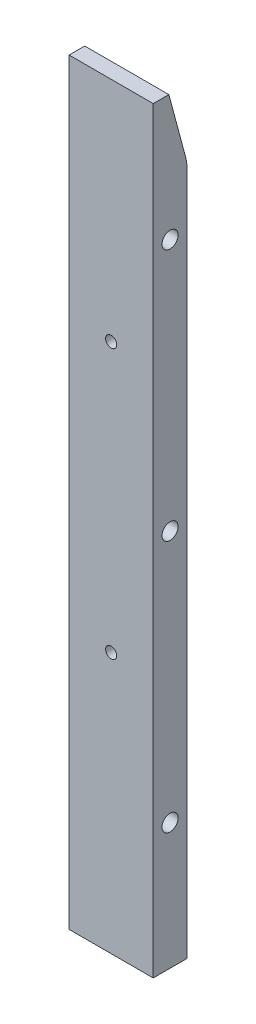
from build123d import *

# Parameters (mm, degrees)
SKETCH_1_W                = 10
SKETCH_1_H                = 225
EXTRUDE_1_DEPTH           = 12.5
CHAMFER_1_SIZE            = 20
CHAMFER_1_SIZE2           = 5.358983849
HOLE_WIZARD_1_D           = 4.8
HOLE_WIZARD_1_CBORE_D     = 8
HOLE_WIZARD_1_CBORE_DEPTH = 5
HOLE_WIZARD_M4_1_D        = 3.3
FILLET_1_R                = 10


with BuildPart() as part:
    # 草图1 → 凸台-拉伸1 (new, symmetric)
    with BuildSketch(Plane(origin=(0, 0, 0), x_dir=(0, 0, -1), z_dir=(1, 0, 0))):
        Rectangle(SKETCH_1_W, SKETCH_1_H)
    extrude(amount=EXTRUDE_1_DEPTH, both=True)

    # 倒角1
    chamfer_1_edges = [part.edges().sort_by_distance(p)[0] for p in [
        (0, 112.5, -5),
    ]]
    chamfer_1_side = [part.faces().sort_by_distance(p)[0] for p in [
        (0, 0, -5),
    ]]
    chamfer(chamfer_1_edges, length=CHAMFER_1_SIZE, length2=CHAMFER_1_SIZE2, reference=chamfer_1_side[0])

    # 打孔尺寸(%根据)开槽圆柱头螺钉的类型1 (through all)
    with Locations(Plane.ZY.offset(12.5)):
        with Locations((0, 75), (0, 0), (0, -75)):
            CounterBoreHole(HOLE_WIZARD_1_D / 2, HOLE_WIZARD_1_CBORE_D / 2, HOLE_WIZARD_1_CBORE_DEPTH)

    # M4 螺纹孔1 (through all)
    with Locations(Plane.XY.offset(5)):
        with Locations((0, 45), (0, -35)):
            Hole(HOLE_WIZARD_M4_1_D / 2)

    # 圆角1
    fillet_1_edges = [part.edges().sort_by_distance(p)[0] for p in [
        (0, 92.5, -5),
    ]]
    fillet(fillet_1_edges, radius=FILLET_1_R)


solid = part.part
